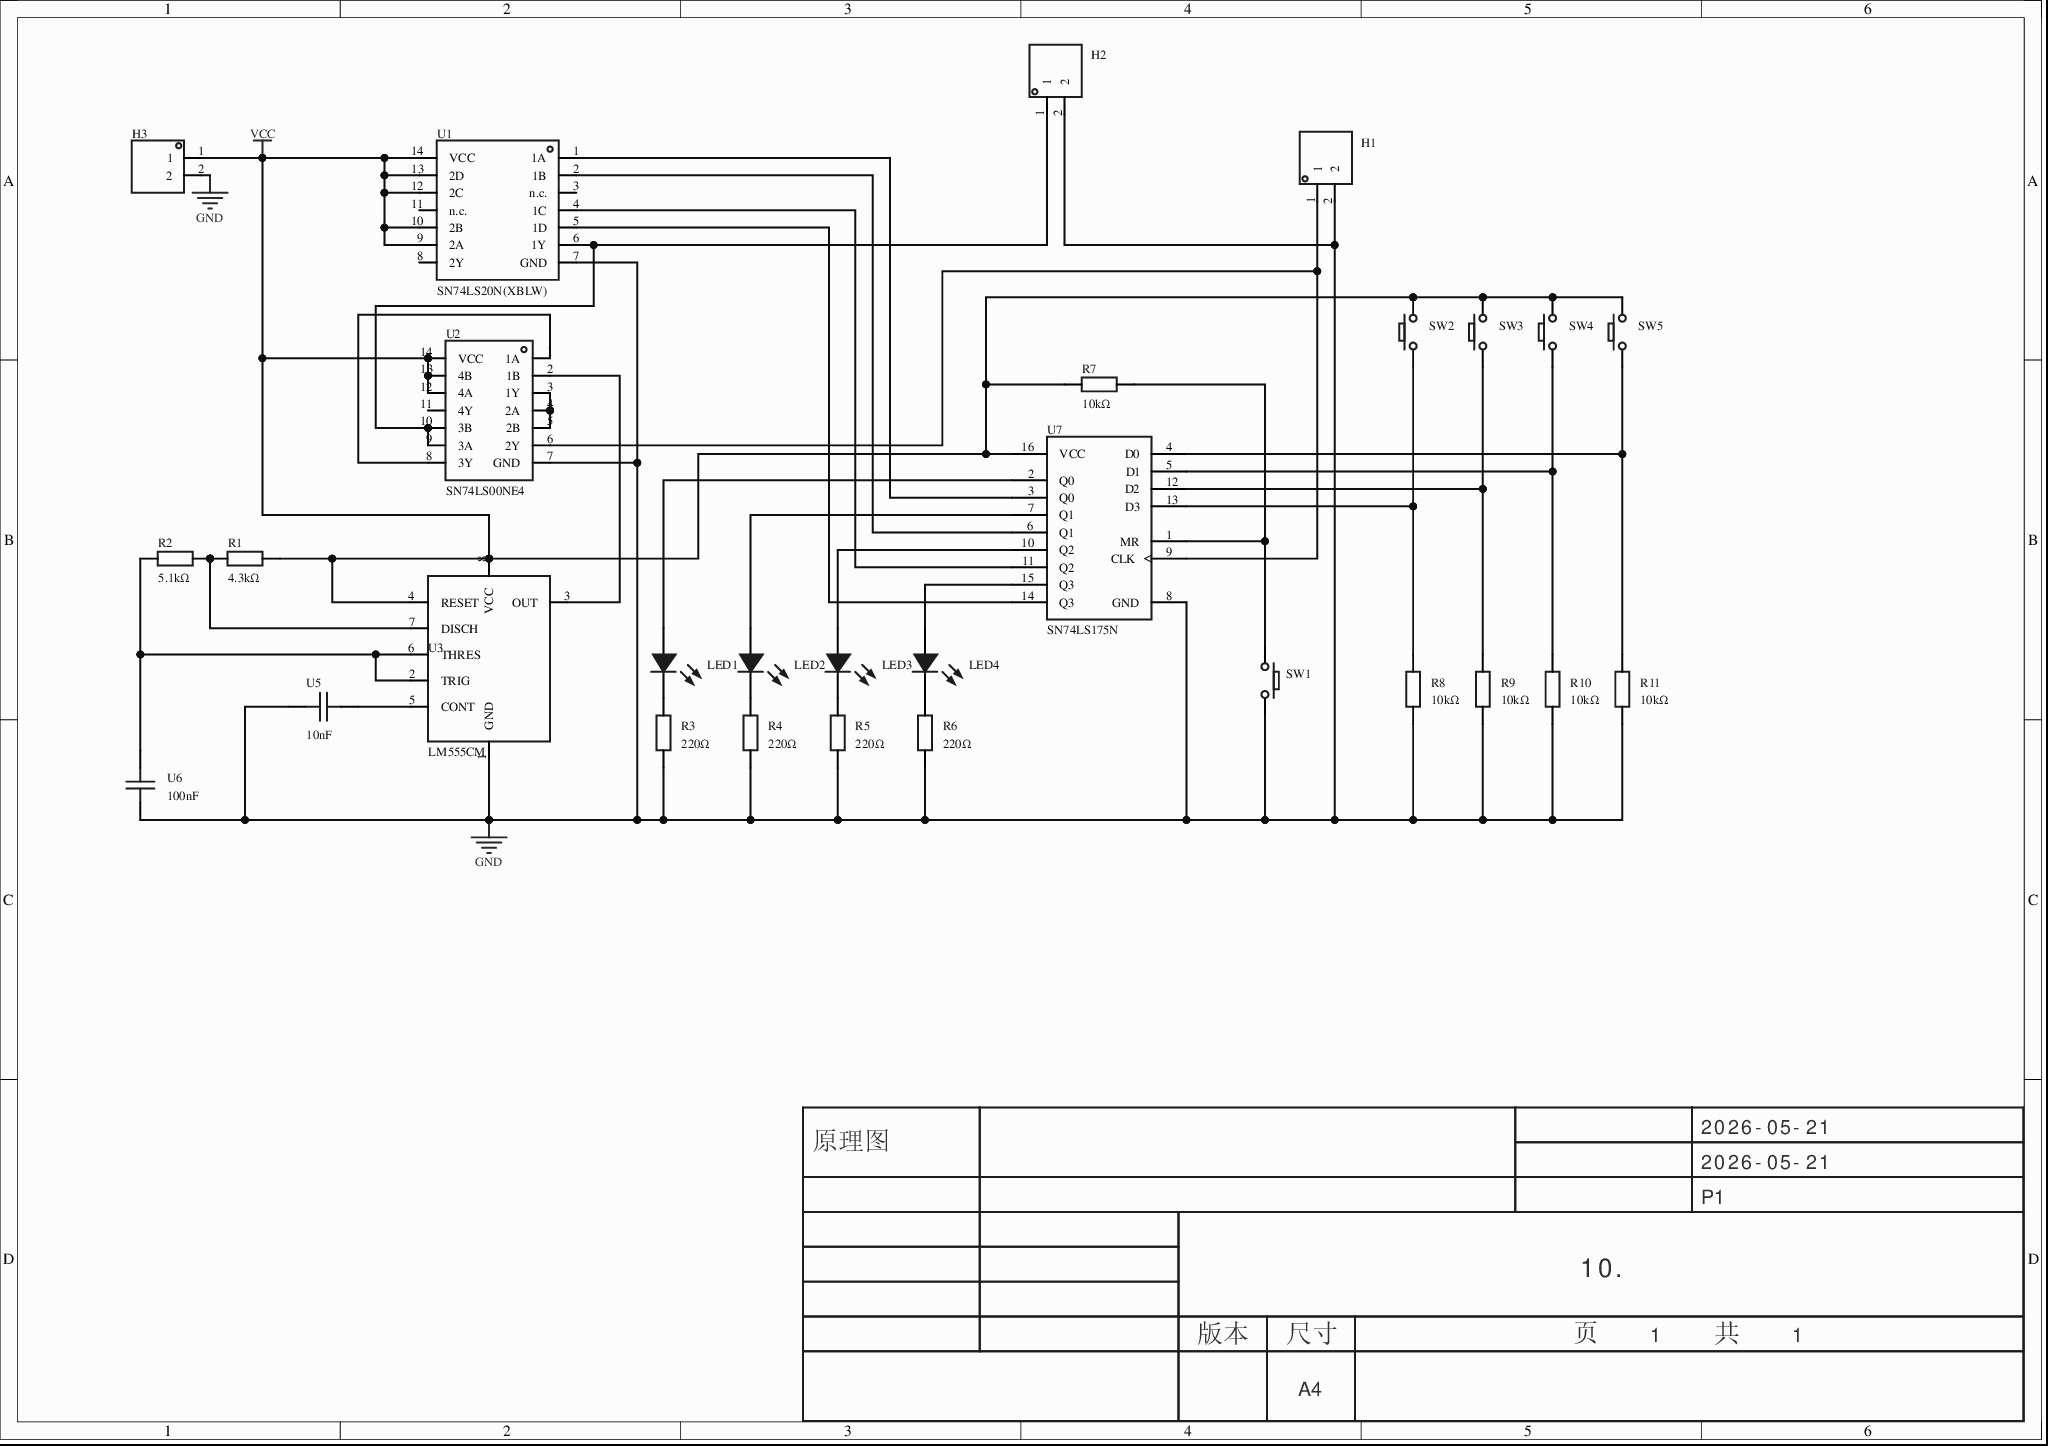
[diagram p0: MISC49856-3.schdoc]
# Altium project MISC49856-2.PrjPcb
1 sheet, 29 parts. Net scope: global (net labels, ports and power ports of the same name join across sheets).
Board file: MISC49856.pcbdoc

## Sheet MISC49856-3.schdoc
size 297 x 209 mm; Version: V1.0; @Project Name: MISC49856; @Update Date: 2026-05-21; @Create Date: 2026-05-21; @Board Name: MISC49856; @Create Time: 21:57:13; @Page Count: 1; @Page No: 1; @Schematic Name: MISC49856; @Update Time: 21:57:13; Size: A4

### Parts
H1  (no value)  [HDR-TH_2P-P2.54-V-M-1]
H2  (no value)  [HDR-TH_2P-P2.54-V-M-1]
H3  (no value)  [HDR-TH_2P-P2.54-V-M-1]
LED1  (no value)  [LED_TH-3mm]
LED2  (no value)  [LED_TH-3mm]
LED3  (no value)  [LED_TH-3mm]
LED4  (no value)  [LED_TH-3mm]
R1  4.3kΩ  [Res_1/8W]
R2  5.1kΩ  [Res_1/8W]
R3  220Ω  [Res_1/8W]
R4  220Ω  [Res_1/8W]
R5  220Ω  [Res_1/8W]
R6  220Ω  [Res_1/8W]
R7  10kΩ  [Res_1/8W]
R8  10kΩ  [Res_1/8W]
R9  10kΩ  [Res_1/8W]
R10  10kΩ  [Res_1/8W]
R11  10kΩ  [Res_1/8W]
SW1  (no value)  [Key_TH_3.5x6x4.3]
SW2  (no value)  [Key_TH_3.5x6x4.3]
SW3  (no value)  [Key_TH_3.5x6x4.3]
SW4  (no value)  [Key_TH_3.5x6x4.3]
SW5  (no value)  [Key_TH_3.5x6x4.3]
U1  SN74LS20N(XBLW)  [DIP-14_L19.0-W6.4-P2.54-LS7.6-BL]
U2  SN74LS00NE4  [PDIP-14_L19.3-W6.4-P2.54-LS7.9-BL]
U3  LM555CM  [PDIP-8_L9.6-W6.4-P2.54-LS7.9-BL-1]
U5  10nF  [CAP-TH_L5.0-W2.5-P5.00-D1.0]
U6  100nF  [CAP-TH_L5.0-W2.5-P5.00-D1.0]
U7  SN74LS175N  [DIP-16_L19.3-W6.4-P2.54-LS7.6-BL]

### Nets
GND: H1.2 H2.2 H3.2 R3.1 R4.1 R5.1 R6.1 R8.1 R9.1 R10.1 R11.1 SW1.A U1.7(GND) U2.7(GND) U3.1(GND) U5.2 U6.2 U7.8(GND)
VCC: H3.1 R1.2 R7.1 SW2.B SW3.B SW4.B SW5.B U1.9(2A) U1.10(2B) U1.12(2C) U1.13(2D) U1.14(VCC) U2.12(4A) U2.13(4B) U2.14(VCC) U3.4(RESET) U3.8(VCC) U7.16(VCC)
NetH1_1: H1.1 U2.6(2Y) U7.9(CLK)
NetH2_1: H2.1 U1.6(1Y) U2.9(3A) U2.10(3B)
NetLED1_1: LED1.1(C) U7.2(Q0)
NetLED1_2: LED1.2(A) R3.2
NetLED2_1: LED2.1(C) U7.7(Q1)
NetLED2_2: LED2.2(A) R4.2
NetLED3_1: LED3.1(C) U7.10(Q2)
NetLED3_2: LED3.2(A) R5.2
NetLED4_1: LED4.1(C) U7.15(Q3)
NetLED4_2: LED4.2(A) R6.2
NetR1_1: R1.1 R2.2 U3.7(DISCH)
NetR2_1: R2.1 U3.2(TRIG) U3.6(THRES) U6.1
NetR7_2: R7.2 SW1.B U7.1(MR)
NetR8_2: R8.2 SW2.A U7.13(D3)
NetR9_2: R9.2 SW3.A U7.12(D2)
NetR10_2: R10.2 SW4.A U7.5(D1)
NetR11_2: R11.2 SW5.A U7.4(D0)
NetU1_1: U1.1(1A) U7.3(Q0)
NetU1_2: U1.2(1B) U7.6(Q1)
NetU1_4: U1.4(1C) U7.11(Q2)
NetU1_5: U1.5(1D) U7.14(Q3)
NetU2_1: U2.1(1A) U2.8(3Y)
NetU2_2: U2.2(1B) U3.3(OUT)
NetU2_3: U2.3(1Y) U2.4(2A) U2.5(2B)
NetU3_5: U3.5(CONT) U5.1

Not connected (* = marked no-connect by the designer): U1 3(n.c.)* 8(2Y)* 11(n.c.)*; U2 11(4Y)*

### Notes on the sheet
- 2026-05-21
- 原理图
- P1
- 10.
- 版本
- 尺寸
- A4
- 页    1    共    1

### Library data of the parts
H1-H3 = HDR-M_2.54_1x2P: Symbol: 210S-1*2P L=11.6MMGold-plated black; ConvertToPcb: yes; ModelId: 79b2e9f2d70a4d68a1b7098f27c6d4c50819f05c4eef4c71ace90d822a990e87; ModelName: HDR-M-2.54_1x2; ModelTransform: 200,100,0,0,0,0,0,0,-118.11; Device: HDR-M_2.54_1x2P; AddInBom: yes; SupplierPart: C124375; Supplier Footprint: 插件; FootprintName: HDR-TH_2P-P2.54-V-M-1
LED1-LED4 = LED_TH-B_3mm: ConvertToPcb: yes; ModelId: ff771fff7070432ca3f353cf0f67af4c0819f05c4eef4c71ace90d822a990e87; ModelName: LED-TH_BD3.8-P2.54-FD_BLUE; ModelTransform: 134.36,149.37,405.47,0,0,0,-11.81,0,-196.85; Symbol: LED_TH-B; Device: LED_TH-B_3mm; AddInBom: yes; Supplier Footprint: 插件; FootprintName: LED_TH-3mm
R1-R11 = Res_AXIAL-1/8W: Symbol: 电阻; ConvertToPcb: yes; ModelId: b2b5ae7ae4c642178fe0039925c86a3f0819f05c4eef4c71ace90d822a990e87; ModelName: RES-TH_BD1.8-L3.2-P7.20-D0.4; ModelTransform: 282.86,66.88,253.09,0,0,0,0,0,-191; Device: Res_AXIAL-1/8W; AddInBom: yes; Supplier Footprint: 轴向引线; FootprintName: Res_1/8W
  R1: Value: 4.3kΩ
  R2: Value: 5.1kΩ
  R3-R6: Value: 220Ω
  R7-R11: Value: 10kΩ
SW1-SW5 = Key_TH_3.5x6x4.3: ConvertToPcb: yes; ModelId: c3523f9014d949d7ba5445190a3178990819f05c4eef4c71ace90d822a990e87; ModelName: SW-TH_L6.0-W3.5-H5.0-P6.5; ModelTransform: 308.49,137.8,335.08,0,0,0,0,0,-129.92; Symbol: Key_TH_3.5x6x4.3; Device: Key_TH_3.5x6x4.3; AddInBom: yes; Supplier Footprint: 插件; FootprintName: Key_TH_3.5x6x4.3
U1 = SN74LS20N(XBLW): 逻辑类型:与非门;通道数:2;工作电压:2V~6V;静态电流(Iq):2uA;传播延迟(tpd):18ns@4.5V；15ns@6V;; Manufacturer: XBLW(芯伯乐); AddInBom: yes; ModelId: 1a65e38672a8476bab35fd02b22b06eb0819f05c4eef4c71ace90d822a990e87; ModelTransform: 748.03,309.842,0,0,0,0,0,0,-125.984; Logic Type: 与非门; Number of Channels: 2; Voltage - Supply: 2V~6V; Quiescent Current: 2uA; Current - Output Low(IOL): 5.2mA; Input Logic Level - High: 1.5V；4.2V；3.15V; Input Logic Level - Low: 500mV；1.35V；1.8V; Output Logic Level - High: 1.9V；5.9V；4.4V; Output Logic Level - Low: 260mV; Input Number: 4; Symbol: SN74LS20N(XBLW); Device: SN74LS20N(XBLW); LCSC Part Name: 双4输入与非门; SupplierPart: C42395510; ManufacturerPart: SN74LS20N(XBLW); Supplier Footprint: DIP-14; JLCPCB Part Class: Extended Part; Datasheet: https://item.szlcsc.com/datasheet/SN74LS20N(XBLW)/44341344.html; Supplier: LCSC; ConvertToPcb: yes; FootprintName: DIP-14_L19.0-W6.4-P2.54-LS7.6-BL; ModelName: DIP-14_L19.0-W6.4-P2.54-LS7.6-BL; Current - Output High(IOH): 5.2mA; Series: 74LS; Propagation Delay: 18ns@4.5V；15ns@6V; Operating Temperature: -20℃~+85℃
U2 = SN74LS00NE4: SN74LS00 4 通道、双输入、4.75V 至 5.25V 双极与非门; Manufacturer: TI(德州仪器); AddInBom: yes; ModelId: ed65e85d32ac41798f005e95ecc59a640819f05c4eef4c71ace90d822a990e87; ModelTransform: 759.841,309.842,0,0,0,0,0,0,-118.11; Symbol: SN74LS00NE4; Device: SN74LS00NE4; LCSC Part Name: SN74LS00NE4; SupplierPart: C20345749; ManufacturerPart: SN74LS00NE4; Supplier Footprint: PDIP-14; JLCPCB Part Class: Extended Part; Datasheet: https://item.szlcsc.com/datasheet/SN74LS00NE4/21671276.html; Supplier: LCSC; ConvertToPcb: yes; FootprintName: PDIP-14_L19.3-W6.4-P2.54-LS7.9-BL; ModelName: PDIP-14_L19.3-W6.4-P2.54-LS7.9-BL
U3 = NE555PE4: NE555 单精度定时器; Manufacturer: TI(德州仪器); Symbol: NE555PE4_1; AddInBom: yes; ModelId: 1b8eaf096e7944deafe216467068c10e0819f05c4eef4c71ace90d822a990e87; ModelTransform: 377.952,318.897,0,0,0,0,0,0,-118.11; Device: NE555PE4; Manufacturer Part: LM555CM; LCSC Part Name: NE555PE4; SupplierPart: C2859604; Supplier Footprint: PDIP-8; JLCPCB Part Class: Extended Part; Datasheet: https://www.ti.com/cn/lit/gpn/sa555; Supplier: LCSC; ConvertToPcb: yes; FootprintName: PDIP-8_L9.6-W6.4-P2.54-LS7.9-BL-1; ModelName: PDIP-8_L9.6-W6.4-P2.54-LS7.9-BL-1
U5 U6 = 100nF: Symbol: 100NF_C9900015256; AddInBom: yes; ModelId: 08e3d7481fc7486bb1b263873f51e1e10819f05c4eef4c71ace90d822a990e87; ModelName: CAP-TH_BD5.0-W2.5-P5.08; ModelTransform: 224.652,98.425,0,0,0,0,-0.005,0,-137.795; Device: 100nF; LCSC Part Name: 100nF; SupplierPart: C9900015256; Supplier Footprint: CAP-TH_L5.0-W2.5-P5.00-D1.0; JLCPCB Part Class: Extended Part; Supplier: LCSC; ConvertToPcb: yes; FootprintName: CAP-TH_L5.0-W2.5-P5.00-D1.0
  U5: Manufacturer Part: 10nF
  U6: Manufacturer Part: 100nF
U7 = SN74LS175N: Symbol: SN74LS175N_1; AddInBom: yes; Device: SN74LS175N; ConvertToPcb: yes